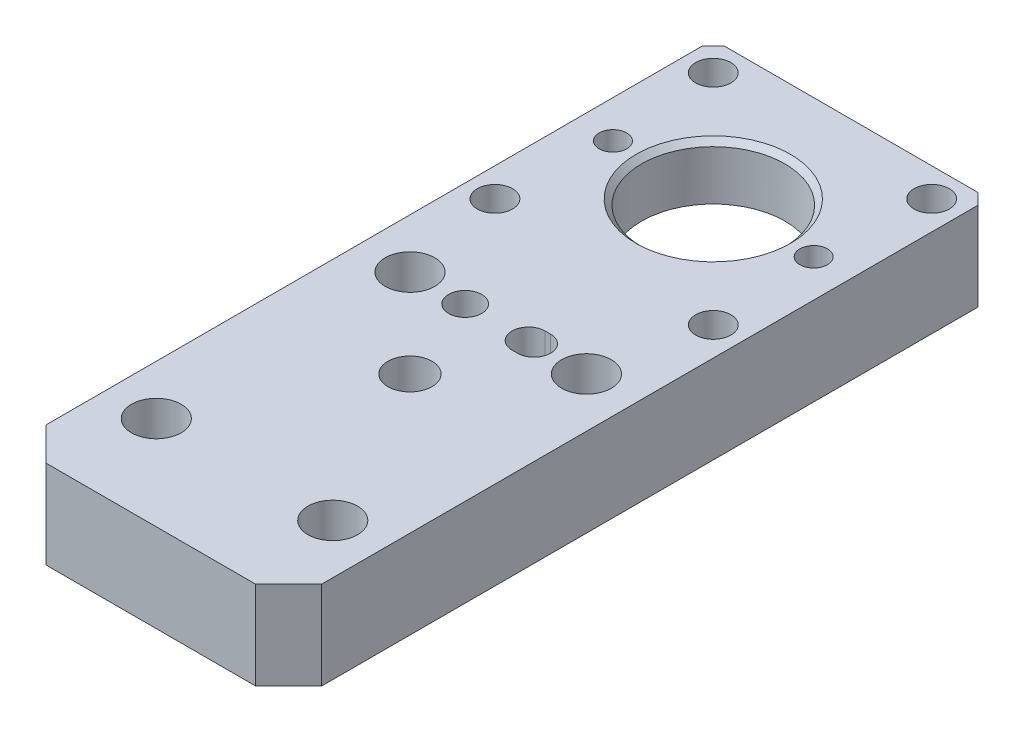
from build123d import *

# Parameters (mm, degrees)
SKETCH1_W                = 25
SKETCH1_H                = 75
BOSS_EXTRUDE1_DEPTH      = 8
SKETCH2_R                = 2.25
CUT_EXTRUDE1_DEPTH       = 20
SKETCH3_R                = 6.5
CUT_EXTRUDE2_DEPTH       = 20
SKETCH4_W                = 35.479601552
SKETCH4_H                = 10
CUT_EXTRUDE3_DEPTH       = 10
SKETCH5_W                = 25
SKETCH5_H                = 6.5
CUT_EXTRUDE4_DEPTH       = 10
CHAMFER1_SIZE            = 3
SKETCH6_R                = 1.6
CUT_EXTRUDE5_DEPTH       = 10
CIRPATTERN1_COUNT        = 4
SKETCH7_R                = 10.25
CUT_EXTRUDE6_DEPTH       = 3
SKETCH8_R                = 2.25
CUT_EXTRUDE7_DEPTH       = 36.72814017
CHAMFER2_SIZE            = 1
F_3_0_3_DIAMETER_HOLE1_D = 3
F_4_0_4_DIAMETER_HOLE1_D = 4
CUT_EXTRUDE8_DEPTH       = 36.72814017
CHAMFER3_SIZE            = 0.5
M3_TAPPED_HOLE1_D        = 2.5
M3_TAPPED_HOLE1_DEPTH    = 8.5
M3_TAPPED_HOLE1_TIP      = 0.751075774


with BuildPart() as part:
    # Sketch1 → Boss-Extrude1 (new body)
    with BuildSketch(Plane(origin=(0, 0, 0), x_dir=(1, 0, 0), z_dir=(0, 1, 0))):
        Rectangle(SKETCH1_W, SKETCH1_H)
    extrude(amount=BOSS_EXTRUDE1_DEPTH)

    # Sketch2 → Cut-Extrude1 (cut)
    with BuildSketch(Plane.XZ):
        with Locations(Location((-8, 24, 0), (0, 0, 270))):
            Circle(SKETCH2_R)
        with Locations(Location((8, 24, 0), (0, 0, 90))):
            Circle(SKETCH2_R)
    extrude(amount=-CUT_EXTRUDE1_DEPTH, mode=Mode.SUBTRACT)

    # Sketch3 → Cut-Extrude2 (cut)
    with BuildSketch(Plane(origin=(0, 8, 0), x_dir=(1, 0, 0), z_dir=(0, 1, 0))):
        with Locations(Location((0, 18.5, 0), (0, 0, 270))):
            Circle(SKETCH3_R)
    extrude(amount=-CUT_EXTRUDE2_DEPTH, mode=Mode.SUBTRACT)

    # Sketch4 → Cut-Extrude3 (cut)
    with BuildSketch(Plane(origin=(0, 8, 0), x_dir=(1, 0, 0), z_dir=(0, 1, 0))):
        with Locations((0, -37.5)):
            Rectangle(SKETCH4_W, SKETCH4_H)
    extrude(amount=-CUT_EXTRUDE3_DEPTH, mode=Mode.SUBTRACT)

    # Sketch5 → Cut-Extrude4 (cut)
    with BuildSketch(Plane(origin=(0, 8, 0), x_dir=(1, 0, 0), z_dir=(0, 1, 0))):
        with Locations((0, 34.25)):
            Rectangle(SKETCH5_W, SKETCH5_H)
    extrude(amount=-CUT_EXTRUDE4_DEPTH, mode=Mode.SUBTRACT)

    # Chamfer1
    chamfer1_edges = [part.edges().sort_by_distance(p)[0] for p in [
        (12.5, 4, 32.5),
        (-12.5, 4, 32.5),
    ]]
    chamfer(chamfer1_edges, length=CHAMFER1_SIZE)

    # Sketch6 → Cut-Extrude5 (cut)
    with BuildSketch(Plane.XZ):
        with Locations(Location((9.899494937, -8.600505063, 0), (0, 0, 270))):
            Circle(SKETCH6_R)
    cut_extrude5 = extrude(amount=-CUT_EXTRUDE5_DEPTH, mode=Mode.SUBTRACT)

    # CirPattern1: Cut-Extrude5 ×4 about axis
    cirpattern1_axis = Axis((0, 0, -18.5), (0, 1, 0))
    for i in range(1, CIRPATTERN1_COUNT):
        add(cut_extrude5.rotate(cirpattern1_axis, i * 360 / CIRPATTERN1_COUNT), mode=Mode.SUBTRACT)

    # Sketch7 → Cut-Extrude6 (cut)
    with BuildSketch(Plane.XZ):
        with Locations(Location((0, -18.5, 0), (0, 0, 270))):
            Circle(SKETCH7_R)
    extrude(amount=-CUT_EXTRUDE6_DEPTH, mode=Mode.SUBTRACT)

    # Sketch8 → Cut-Extrude7 (cut, through all)
    with BuildSketch(Plane(origin=(0, 8, 0), x_dir=(1, 0, 0), z_dir=(0, 1, 0))):
        with Locations(Location((-8, -1, 0), (0, 0, 270))):
            Circle(SKETCH8_R)
        with Locations(Location((8, -1, 0), (0, 0, 90))):
            Circle(SKETCH8_R)
    extrude(amount=-CUT_EXTRUDE7_DEPTH, mode=Mode.SUBTRACT)

    # Chamfer2
    chamfer2_edges = [part.edges().sort_by_distance(p)[0] for p in [
        (-12.5, 4, -31),
        (12.5, 4, -31),
    ]]
    chamfer(chamfer2_edges, length=CHAMFER2_SIZE)

    # Ø3.0 (3) Diameter Hole1 (through all)
    with Locations(Plane(origin=(0, 0, 0), x_dir=(-1, 0, 0), z_dir=(0, -1, 0))):
        with Locations((3, -1), (-3, -1)):
            Hole(F_3_0_3_DIAMETER_HOLE1_D / 2)

    # Ø4.0 (4) Diameter Hole1 (through all)
    with Locations(Plane(origin=(0, 0, 0), x_dir=(-1, 0, 0), z_dir=(0, -1, 0))):
        with Locations((0, -9)):
            Hole(F_4_0_4_DIAMETER_HOLE1_D / 2)

    # Sketch14 → Cut-Extrude8 (cut, through all)
    with BuildSketch(Plane(origin=(0, 8, 0), x_dir=(1, 0, 0), z_dir=(0, 1, 0))):
        with BuildLine():
            Line((2.75, 0.5), (3.25, 0.5))
            ThreePointArc((3.25, 0.5), (4.75, -1), (3.25, -2.5))
            Line((3.25, -2.5), (2.75, -2.5))
            ThreePointArc((2.75, -2.5), (1.25, -1), (2.75, 0.5))
        make_face()
    extrude(amount=-CUT_EXTRUDE8_DEPTH, mode=Mode.SUBTRACT)

    # Chamfer3
    chamfer3_edges = [part.edges().sort_by_distance(p)[0] for p in [
        (0, 0, -8.25),
        (0, 8, -25),
    ]]
    chamfer(chamfer3_edges, length=CHAMFER3_SIZE)

    # M3 Tapped Hole1
    with Locations(Plane(origin=(0, 8, 0), x_dir=(1, 0, 0), z_dir=(0, 1, 0))):
        with Locations((-9.1, 18.5), (9.1, 18.5)):
            Hole(M3_TAPPED_HOLE1_D / 2, depth=M3_TAPPED_HOLE1_DEPTH)
            with Locations((0, 0, -(M3_TAPPED_HOLE1_DEPTH + M3_TAPPED_HOLE1_TIP / 2))):  # 118° drill point
                Cone(0, M3_TAPPED_HOLE1_D / 2, M3_TAPPED_HOLE1_TIP, mode=Mode.SUBTRACT)


solid = part.part
